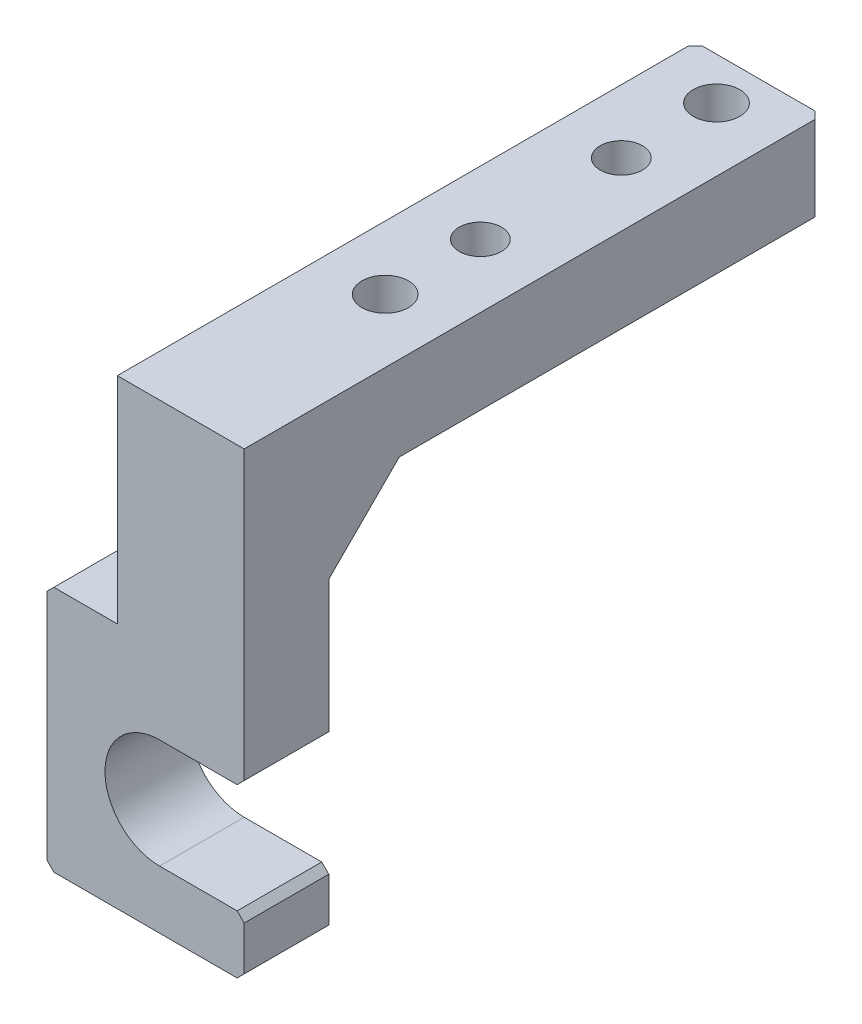
from build123d import *

# Parameters (mm, degrees)
SKETCH_1_W                   = 18
SKETCH_1_H                   = 65.5
EXTRUDE_1_DEPTH              = 6
SKETCH_2_W                   = 28
SKETCH_2_H                   = 35
EXTRUDE_2_DEPTH              = 12
CUT_EXTRUDE_1_DEPTH          = 40.71854101
SKETCH_4_W                   = 18
SKETCH_4_H                   = 12
EXTRUDE_3_DEPTH              = 70
CHAMFER_1_SIZE               = 10
HOLE_WIZARD_M6_1_D           = 6.6
HOLE_WIZARD_M6_1_CBORE_D     = 11
HOLE_WIZARD_M6_1_CBORE_DEPTH = 6.4
F_6_0MM_1_D                  = 6
CHAMFER_2_SIZE               = 1


with BuildPart() as part:
    # 草图1 → 凸台-拉伸1 (new, symmetric)
    with BuildSketch(Plane.XY):
        Rectangle(SKETCH_1_W, SKETCH_1_H)
    extrude(amount=EXTRUDE_1_DEPTH, both=True)

    # 草图2 → 凸台-拉伸2 (add)
    with BuildSketch(Plane.XY.offset(6)):
        with Locations((-5, -15.25)):
            Rectangle(SKETCH_2_W, SKETCH_2_H)
    extrude(amount=-EXTRUDE_2_DEPTH)

    # 草图3 → 切除-拉伸1 (cut, through all)
    with BuildSketch(Plane.XY.offset(6)):
        with BuildLine():
            Line((-3, -9), (21, -9))
            ThreePointArc((21, -9), (28.75, -16.75), (21, -24.5))
            Line((21, -24.5), (-3, -24.5))
            ThreePointArc((-3, -24.5), (-10.75, -16.75), (-3, -9))
        make_face()
    extrude(amount=-CUT_EXTRUDE_1_DEPTH, mode=Mode.SUBTRACT)

    # 草图4 → 凸台-拉伸3 (add)
    with BuildSketch(Plane(origin=(0, 0, -6), x_dir=(-1, 0, 0), z_dir=(0, 0, -1))):
        with Locations((0, 26.75)):
            Rectangle(SKETCH_4_W, SKETCH_4_H)
    extrude(amount=EXTRUDE_3_DEPTH)

    # 倒角1
    chamfer_1_edges = [part.edges().sort_by_distance(p)[0] for p in [
        (0, 20.75, -6),
    ]]
    chamfer(chamfer_1_edges, length=CHAMFER_1_SIZE)

    # M6 六角凹头螺钉的柱形沉头孔1 (through all)
    with Locations(Plane(origin=(0, 20.75, 0), x_dir=(-1, 0, 0), z_dir=(0, -1, 0))):
        with Locations((0, 23), (0, 70)):
            CounterBoreHole(HOLE_WIZARD_M6_1_D / 2, HOLE_WIZARD_M6_1_CBORE_D / 2, HOLE_WIZARD_M6_1_CBORE_DEPTH)

    # Ø6.0mm 暗销孔1 (through all)
    with Locations(Plane(origin=(0, 20.75, 0), x_dir=(-1, 0, 0), z_dir=(0, -1, 0))):
        with Locations((0, 36.5), (0, 56.5)):
            Hole(F_6_0MM_1_D / 2)

    # 倒角2
    chamfer_2_edges = [part.edges().sort_by_distance(p)[0] for p in [
        (-19, 2.25, 0),
        (-19, -32.75, 0),
        (9, -9, 0),
        (9, -24.5, 0),
        (-9, 26.75, -76),
        (9, 26.75, -76),
        (9, -32.75, 0),
    ]]
    chamfer(chamfer_2_edges, length=CHAMFER_2_SIZE)


solid = part.part
